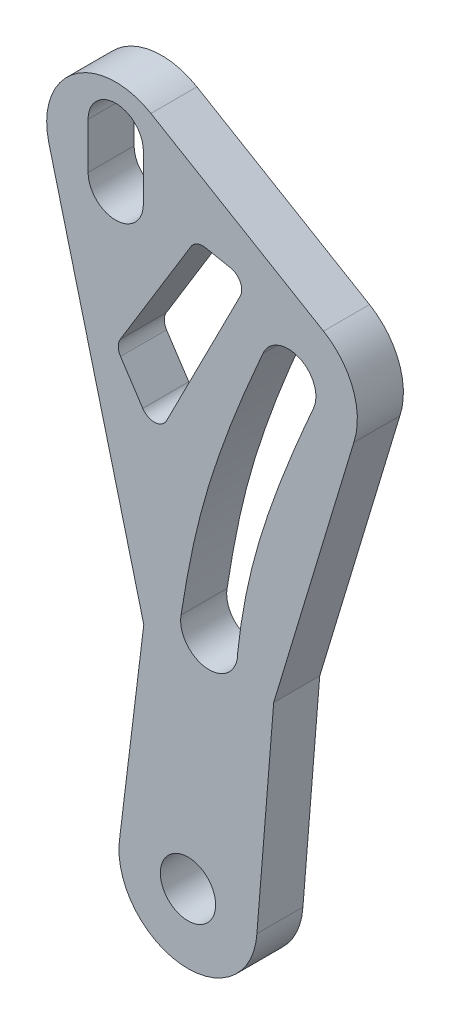
SolidWorks part; units mm, degrees
ref_plane "Front Plane" through (0, 0, 0) normal (0, 0, 1) x (1, 0, 0)
ref_plane "Top Plane" through (0, 0, 0) normal (0, 1, 0) x (1, 0, 0)
ref_plane "Right Plane" through (0, 0, 0) normal (1, 0, 0) x (0, 0, -1)
sketch "Sketch1" plane through (0, 0, 0) normal (0, 0, 1) x (1, 0, 0)
  line L0 (0, 0) -> (0, 170)
  line L1 (0, 170) -> (100, 170)
  line L2 (100, 170) -> (100, 0)
  line L4 (0, 0) -> (0, -20)
  line L5 (0, -20) -> (100, -20)
  line L6 (100, -20) -> (100, 0)
extrude "Boss-Extrude1" add sketch "Sketch1" along normal blind 10
sketch "Sketch6" plane through (0, 0, 10) normal (0, 0, 1) x (1, 0, 0)
  circle A0 centre (50, -5) radius 6
sketch "Sketch9" plane through (0, 0, 10) normal (0, 0, 1) x (1, 0, 0)
  line L1 (29.7878, 148.9088) -> (29.7878, 138.9088)
  line L2 (41.7878, 148.9088) -> (41.7878, 138.9088)
  arc A0 (29.7878, 138.9088) -> (41.7878, 138.9088) centre (35.7878, 138.9088) ccw
  arc A1 (41.7878, 148.9088) -> (29.7878, 148.9088) centre (35.7878, 148.9088) ccw
sketch "Sketch10" plane through (0, 0, 10) normal (0, 0, 1) x (1, 0, 0)
  circle A0 centre (35.7878, 139.9121) radius 6
extrude "Cut-Extrude8" cut sketch "Sketch9" against normal blind 10 contours A1 L1 A0 L2
sketch "Sketch21" plane through (0, 0, 0) normal (0, 0, -1) x (-1, 0, 0)
  circle A0 centre (-51.4832, 14.9449) radius 6
  circle A1 centre (-173.1256, 5.8991) radius 6
extrude "Cut-Extrude14" cut sketch "Sketch21" against normal blind 36
sketch "Sketch22" plane through (0, 0, 10) normal (0, 0, 1) x (1, 0, 0)
  circle A0 centre (56.0921, 64.6809) radius 6.2
sketch "Sketch23" plane through (0, 0, 10) normal (0, 0, 1) x (1, 0, 0)
  circle A0 centre (73.2683, 121.4516) radius 6
sketch "Sketch24" plane through (0, 0, 10) normal (0, 0, 1) x (1, 0, 0)
  circle A0 centre (63.4898, 96.7917) radius 6
sketch "Sketch25" plane through (0, 0, 10) normal (0, 0, 1) x (1, 0, 0)
  circle A0 centre (60.0061, 85.2501) radius 6
sketch "Sketch28" plane through (0, 0, 10) normal (0, 0, 1) x (1, 0, 0)
  circle A0 centre (73.2683, 121.4516) radius 6 construction
  circle A5 centre (56.0921, 64.6809) radius 6.2 construction
  arc A6 (78.7966, 119.1195) -> (67.7401, 123.7837) centre (73.2683, 121.4516) ccw
  arc A7 (49.9838, 65.7431) -> (62.2889, 64.8821) centre (56.0921, 64.6809) ccw
  spline S0 degree 3 poles (67.7401, 123.7837) (64.0923, 115.4801) (59.1095, 103.3695) (53.1618, 83.9401) (51.1006, 72.8759) (49.9838, 65.7431) knots 0 0 0 0 0.446952 0.644101 1 1 1 1
  spline S1 degree 3 poles (78.7966, 119.1195) (75.2302, 110.9371) (70.2528, 99.0335) (65.5914, 83.7502) (63.4594, 73.9239) (62.6024, 67.8828) (62.2889, 64.8821) knots 0 0 0 0 0.4577 0.660132 0.817977 0.972547 0.972547 0.972547 0.972547
extrude "Cut-Extrude15" cut sketch "Sketch28" against normal blind 10
sketch "Sketch29" plane through (0, 0, 10) normal (0, 0, 1) x (1, 0, 0)
  circle A1 centre (51.4832, 14.9449) radius 15
sketch "Sketch19" plane through (0, 0, 10) normal (0, 0, 1) x (1, 0, 0)
  line L0 (41.8818, 59.8782) -> (36.6898, 17.4262)
  line L1 (21.2005, 140.4141) -> (41.326, 62.0425)
  line L3 (43.4327, 156.8144) -> (80.9252, 134.6048)
  line L4 (87.5081, 116.9486) -> (70.725, 61.3826)
  line L6 (70.1042, 59.3273) -> (66.4544, 14.0169)
  line L7 (41.326, 62.0425) -> (41.8818, 59.8782)
  line L8 (70.725, 61.3826) -> (70.1042, 59.3273)
  line L9 (52.1212, 136.108) -> (36.7797, 111.0157)
  line L10 (36.8317, 107.8039) -> (41.6626, 100.4488)
  line L11 (46.8432, 100.7339) -> (62.8279, 132.1117)
  line L12 (60.7301, 136.4178) -> (55.256, 137.4875)
  arc A2 (36.6898, 17.4262) -> (66.4544, 14.0169) centre (51.4832, 14.9449) ccw
  arc A3 (43.4327, 156.8144) -> (21.2005, 140.4141) centre (35.7878, 143.9088) ccw
  arc A4 (87.5081, 116.9486) -> (80.9252, 134.6048) centre (73.2802, 121.6992) ccw
  circle A6 centre (58.773, 71.2419) radius 125.5172
  arc A7 (36.8317, 107.8039) -> (36.7797, 111.0157) centre (39.3392, 109.4509) cw
  arc A8 (41.6626, 100.4488) -> (46.8432, 100.7339) centre (44.1701, 102.0957) ccw
  arc A9 (62.8279, 132.1117) -> (60.7301, 136.4178) centre (60.1548, 133.4735) ccw
  arc A10 (55.256, 137.4875) -> (52.1212, 136.108) centre (54.6807, 134.5431) ccw
  dimension "D1" = 3
extrude "Cut-Extrude16" cut sketch "Sketch19" against normal blind 10 contours L12 A10 L9 A7 L10 A8 L11 A9 | A6 | L1 L7 L0 A2 L6 L8 L4 A4 L3 A3
